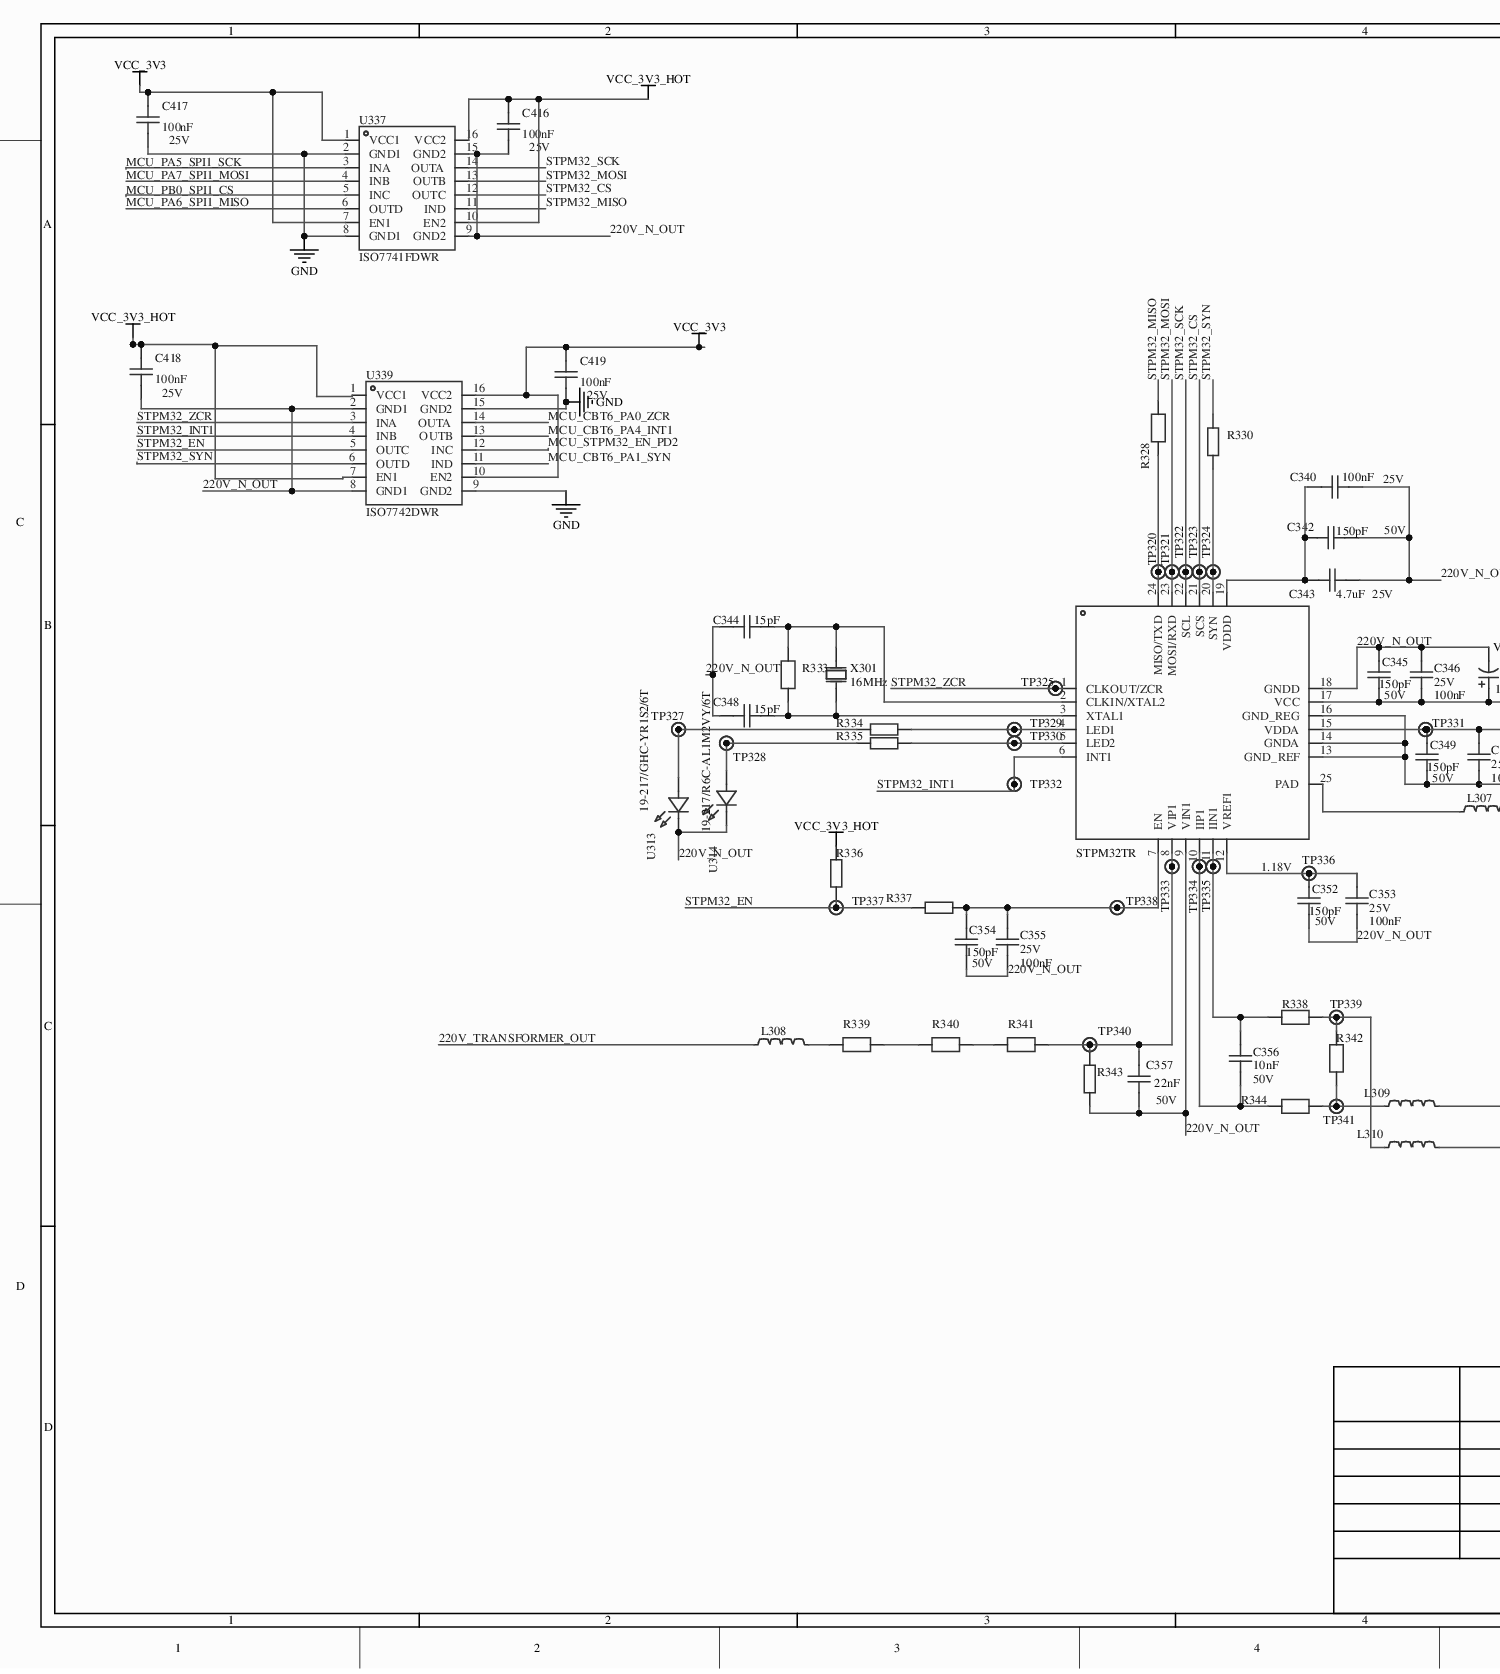
[diagram p0: MISC84429-5.SchDoc, left]
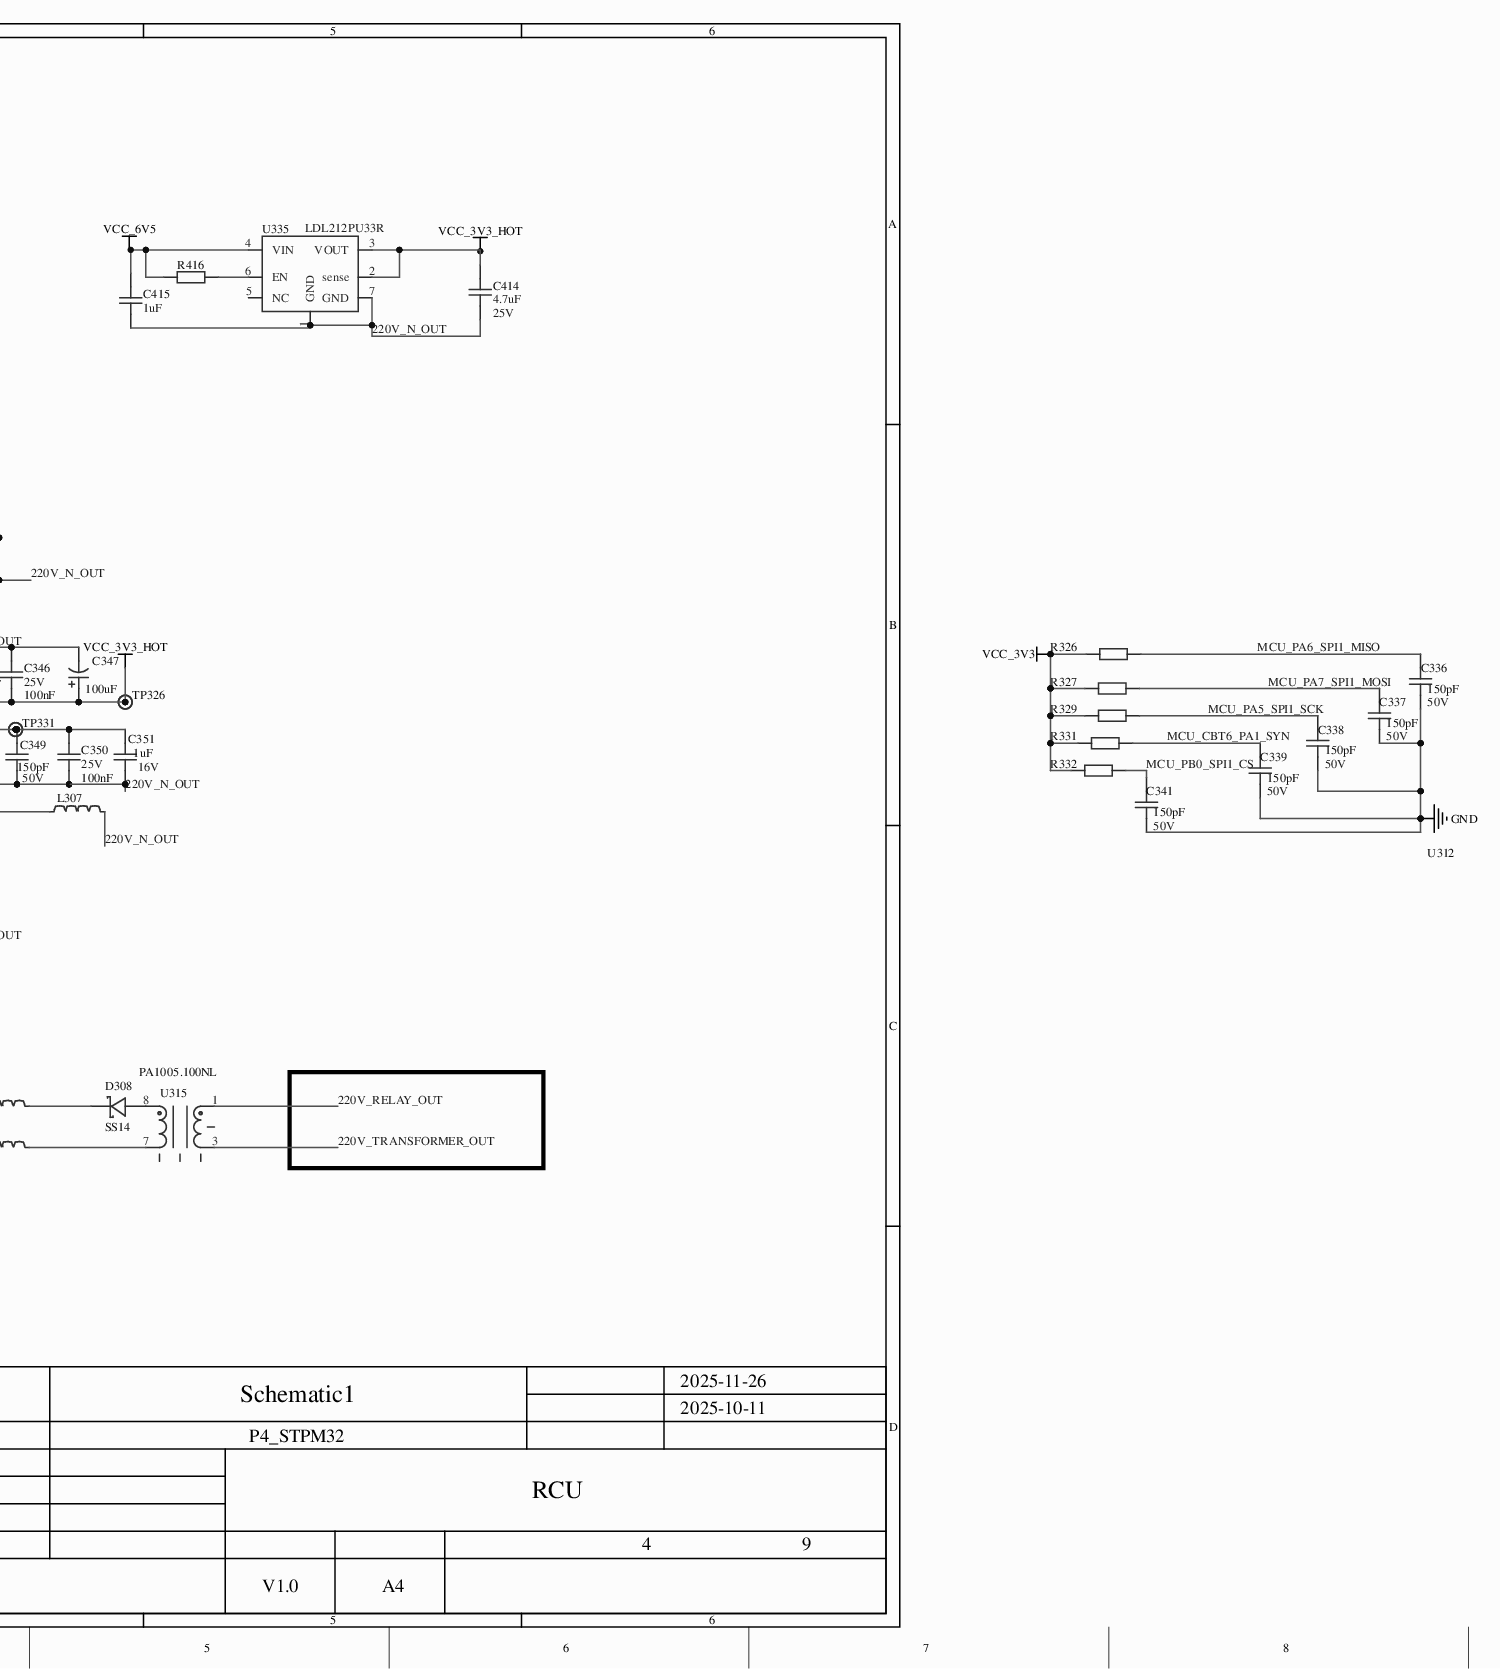
[diagram p1: MISC84429-5.SchDoc, right]
# Altium project MISC84429-12.PrjPcb (part 3 of 5)

## Sheet MISC84429-5.SchDoc
size A1; Name: Sheet-Symbol; Symbol: Sheet-Symbol; Device: Sheet-Symbol; @Page No: 4; @Page Count: 9; @Schematic Name: 1_P1; @Project Name: Altium_Altium_RCU_2025-11-28_2026-01-14; @Board Name: 1_P1; @Update Date: 2026-01-15; @Create Time: 06:40:55; @Update Time: 14:40:57; @Page Name: 4_P4_STPM32; @Create Date: 2026-01-15

### Parts
C336  150pF  Voltage Rating: 50V  [C0603]
C337  150pF  Voltage Rating: 50V  [C0603]
C338  150pF  Voltage Rating: 50V  [C0603]
C339  150pF  Voltage Rating: 50V  [C0603]
C340  100nF  Voltage Rated: 25V  [C0603]
C341  150pF  Voltage Rating: 50V  [C0603]
C342  150pF  Voltage Rating: 50V  [C0603]
C343  4.7uF  Voltage Rating: 25V  [C0603]
C344  15pF  [C0603]
C345  150pF  Voltage Rating: 50V  [C0603]
C346  100nF  Voltage Rated: 25V  [C0603]
C347  100uF  [CAP-SMD_BD6.3-L6.6-W6.6-LS7.3-FD-H7.7]
C348  15pF  [C0603]
C349  150pF  Voltage Rating: 50V  [C0603]
C350  100nF  Voltage Rated: 25V  [C0603]
C351  1uF  Voltage Rated: 16V  [C0603]
C352  150pF  Voltage Rating: 50V  [C0603]
C353  100nF  Voltage Rated: 25V  [C0603]
C354  150pF  Voltage Rating: 50V  [C0603]
C355  100nF  Voltage Rated: 25V  [C0603]
C356  10nF  Voltage Rating: 50V  [C0603]
C357  22nF  Voltage Rating: 50V  [C0805]
C414  4.7uF  Voltage Rating: 25V  [C0603]
C415  1uF  [C0603]
C416  100nF  Voltage Rated: 25V  [C0603]
C417  100nF  Voltage Rated: 25V  [C0603]
C418  100nF  Voltage Rated: 25V  [C0603]
C419  100nF  Voltage Rated: 25V  [C0603]
D308  SS14  [SMA_L4.3-W2.6-LS5.2-RD]
L307  (no value)  [L0805]
L308  (no value)  [L0805]
L309  (no value)  [L0805]
L310  (no value)  [L0805]
R326  (no value)  [R0603]
R327  (no value)  [R0603]
R328  (no value)  [R0603]
R329  (no value)  [R0603]
R330  (no value)  [R0603]
R331  (no value)  [R0603]
R332  (no value)  [R0603]
R333  (no value)  [R0603]
R334  (no value)  [R0603]
R335  (no value)  [R0603]
R336  (no value)  [R0603]
R337  (no value)  [R0603]
R338  (no value)  [R1206]
R339  (no value)  [R1206]
R340  (no value)  [R1206]
R341  (no value)  [R1206]
R342  (no value)  [R1206]
R343  (no value)  [R1206]
R344  (no value)  [R1206]
R416  (no value)  [R0603]
TP320  (no value)  [Test-Point-0.5mm]
TP321  (no value)  [Test-Point-0.5mm]
TP322  (no value)  [Test-Point-0.5mm]
TP323  (no value)  [Test-Point-0.5mm]
TP324  (no value)  [Test-Point-0.5mm]
TP325  (no value)  [Test-Point-0.5mm]
TP326  (no value)  [Test-Point-0.5mm]
TP327  (no value)  [Test-Point-0.5mm]
TP328  (no value)  [Test-Point-0.5mm]
TP329  (no value)  [Test-Point-0.5mm]
TP330  (no value)  [Test-Point-0.5mm]
TP331  (no value)  [Test-Point-0.5mm]
TP332  (no value)  [Test-Point-0.5mm]
TP333  (no value)  [Test-Point-0.5mm]
TP334  (no value)  [Test-Point-0.5mm]
TP335  (no value)  [Test-Point-0.5mm]
TP336  (no value)  [Test-Point-0.5mm]
TP337  (no value)  [Test-Point-0.5mm]
TP338  (no value)  [Test-Point-0.5mm]
TP339  (no value)  [Test-Point-0.5mm]
TP340  (no value)  [Test-Point-0.5mm]
TP341  (no value)  [Test-Point-0.5mm]
U312  STPM32TR  [VQFN-24_L4.0-W4.0-P0.50-BL-EP2.3]
U313  19-217/GHC-YR1S2/6T  [LED0603-RD_GREEN]
U314  19-217/R6C-AL1M2VY/6T  [LED0603-R-FD]
U315  PA1005.100NL  [SENSOR-TH_PA1005.100NL]
U335  LDL212PU33R  [VSON-6_L3.0-W3.0-P0.95-TL-EP_TI_DRP]
U337  ISO7741FDWR  [SOIC-16_L10.3-W7.5-P1.27-LS10.3-BL]
U339  ISO7742DWR  [SOIC-16_L10.3-W7.5-P1.27-LS10.3-BL]
X301  16MHz  [CRYSTAL-SMD_2P-L5.0-W3.2]

### Nets
GND: C336.2 C337.2 C338.2 C339.2 C341.2 C417.2 C419.2 U337.2(GND1) U337.8(GND1) U339.9(GND2) U339.15(GND2)
VCC_3V3: C417.1 C419.1 R326.1 R327.1 R329.1 R331.1 R332.1 U337.1(VCC1) U337.7(EN1) U339.10(EN2) U339.16(VCC2)
VCC_3V3_HOT: C345.1 C346.1 C347.1 C414.2 C416.1 C418.1 R336.2 TP326.1 U312.17(VCC) U335.2(sense) U335.3(VOUT) U337.10(EN2) U337.16(VCC2) U339.1(VCC1) U339.7(EN1)
VCC_6V5: C415.2 R416.1 U335.4(VIN)
220V_N_OUT: C340.2 C342.2 C343.1 C344.1 C345.2 C346.2 C347.2 C348.1 C349.1 C350.1 C351.1 C352.1 C353.1 C354.1 C355.1 C357.1 C414.1 C415.1 C416.2 C418.2 L307.2 R343.1 U312.9(VIN1) U312.13(GND_REF) U312.14(GNDA) U312.16(GND_REG) U312.18(GNDD) U313.1(K) U314.2(K) U335.1(GND) U335.7(GND) U337.9(GND2) U337.15(GND2) U339.2(GND1) U339.8(GND1)
220V_RELAY_OUT: U315.1
220V_TRANSFORMER_OUT: L308.1 U315.3
MCU_CBT6_PA0_ZCR: U339.14(OUTA)
MCU_CBT6_PA1_SYN: C339.1 R331.2 U339.11(IND)
MCU_CBT6_PA4_INT1: U339.13(OUTB)
MCU_PA5_SPI1_SCK: C338.1 R329.2 U337.3(INA)
MCU_PA6_SPI1_MISO: C336.1 R326.2 U337.6(OUTD)
MCU_PA7_SPI1_MOSI: C337.1 R327.2 U337.4(INB)
MCU_PB0_SPI1_CS: C341.1 R332.2 U337.5(INC)
MCU_STPM32_EN_PD2: U339.12(INC)
STPM32_CS: TP323.1 U312.21(SCS) U337.12(OUTC)
STPM32_EN: R336.1 R337.2 TP337.1 U339.5(OUTC)
STPM32_INT1: TP332.1 U312.6(INT1) U339.4(INB)
STPM32_MISO: R328.2 U337.11(IND)
STPM32_MOSI: TP321.1 U312.23(MOSI/RXD) U337.13(OUTB)
STPM32_SCK: TP322.1 U312.22(SCL) U337.14(OUTA)
STPM32_SYN: R330.2 U339.6(OUTD)
STPM32_ZCR: TP325.1 U312.1(CLKOUT/ZCR) U339.3(INA)
NetC340_1: C340.1 C342.1 C343.2 U312.19(VDDD)
NetC344_2: C344.2 R333.2 U312.2(CLKIN/XTAL2) X301.2(OSC2)
NetC348_2: C348.2 R333.1 U312.3(XTAL1) X301.1(OSC1)
NetC349_2: C349.2 C350.2 C351.2 TP331.1 U312.15(VDDA)
NetC352_2: C352.2 C353.2 TP336.1 U312.12(VREF1)
NetC354_2: C354.2 C355.2 R337.1 TP338.1 U312.7(EN)
NetC356_1: C356.1 R344.1 TP334.1 U312.10(IIP1)
NetC356_2: C356.2 R338.1 TP335.1 U312.11(IIN1)
NetC357_2: C357.2 R341.1 R343.2 TP333.1 TP340.1 U312.8(VIP1)
NetD308_1: D308.1(K) L309.2
NetD308_2: D308.2(A) U315.8
NetL307_1: L307.1 U312.25(PAD)
NetL308_2: L308.2 R339.2
NetL309_1: L309.1 R342.1 R344.2 TP341.1
NetL310_1: L310.1 R338.2 R342.2 TP339.1
NetL310_2: L310.2 U315.7
NetR328_1: R328.1 TP320.1 U312.24(MISO/TXD)
NetR330_1: R330.1 TP324.1 U312.20(SYN)
NetR334_1: R334.1 TP327.1 U313.2(A)
NetR334_2: R334.2 TP329.1 U312.4(LED1)
NetR335_1: R335.1 TP328.1 U314.1(A)
NetR335_2: R335.2 TP330.1 U312.5(LED2)
NetR339_1: R339.1 R340.1
NetR340_2: R340.2 R341.2
NetR416_2: R416.2 U335.6(EN)

Not connected (* = marked no-connect by the designer): U315 2* 4* 5* 6*; U335 5(NC)*

### Notes on the sheet
- 1.18V
- 1
- 2
- 3
- 4
- 5
- 6
- A
- B
- C
- D
- Schematic1
- 2025-11-26
- 2025-10-11
- P4_STPM32
- RCU
- 9
- V1.0
- A4

### Library data of the parts
C336-C339 C341 C342 C345 C349 C352 C354 = 150pF: Symbol: GRM1885C1H151JA01D; Add into BOM: yes; Temperature Coefficient: C0G; Device: 150pF; Supplier Part: C85975; Manufacturer Part: GRM1885C1H151JA01D; Supplier Footprint: 0603; Datasheet: https://item.szlcsc.com/datasheet/GRM1885C1H151JA01D/87151.html; Supplier: LCSC; Convert to PCB: yes; Value: 150pF; Origin Footprint: C0603; Design Item ID: GRM1885C1H151JA01D
C340 C346 C350 C353 C355 = 100nF: Symbol: GRM188R71E104KA01D; Add into BOM: yes; Temperature Coefficient: X7R; Device: 100nF; Supplier Part: C77050; Manufacturer Part: GRM188R71E104KA01D; Supplier Footprint: 0603; Datasheet: https://atta.szlcsc.com/upload/public/pdf/source/20170622/1498103881034.pdf; Supplier: LCSC; Convert to PCB: yes; Value: 100nF; Origin Footprint: C0603; Design Item ID: GRM188R71E104KA01D
C343 = 4.7uF: Symbol: GRM188R61E475KE11D; Add into BOM: yes; Temperature Coefficient: X5R; Device: 4.7uF; Supplier Part: C90057; Manufacturer Part: GRM188R61E475KE11D; Supplier Footprint: 0603; Datasheet: https://item.szlcsc.com/datasheet/GRM188R61E475KE11D/91242.html; Supplier: LCSC; Convert to PCB: yes; Value: 4.7uF; Origin Footprint: C0603; Design Item ID: GRM188R61E475KE11D
C344 C348 = 15pF: Symbol: GRM1885C1H150JA01D; Add into BOM: yes; Voltage Rated: 50V; Temperature Coefficient: C0G; Device: 15pF; Supplier Part: C71651; Manufacturer Part: GRM1885C1H150JA01D; Supplier Footprint: 0603; Datasheet: https://atta.szlcsc.com/upload/public/pdf/source/20170116/1484561236820.pdf; Supplier: LCSC; Convert to PCB: yes; Value: 15pF; Origin Footprint: C0603; Design Item ID: GRM1885C1H150JA01D
C347 = 100uF: Symbol: JVJ50V100M6x8; Add into BOM: yes; Voltage Rating: 50V; Ripple Current: 140mA@120Hz; Device: 100uF; Supplier Part: C46550415; Manufacturer Part: JVJ50V100M6x8; Supplier Footprint: SMD,D6.3xL7.7mm; Datasheet: https://item.szlcsc.com/datasheet/JVJ50V100M6x8/48680109.html; Supplier: LCSC; Convert to PCB: yes; Value: 100uF; Diameter: 6.3mm; Height - Seated (Max): 7.7mm; Origin Footprint: CAP-SMD_BD6.3-L6.6-W6.6-LS7.3-FD-H7.7; Design Item ID: JVJ50V100M6x8
C351 = 1uF: Symbol: GCM188R71C105KA64D; Add into BOM: yes; Temperature Coefficient: X7R; Device: 1uF; Supplier Part: C161212; Manufacturer Part: GCM188R71C105KA64D; Supplier Footprint: 0603; Datasheet: https://atta.szlcsc.com/upload/public/pdf/source/20181221/C161212_C96DD77354D5551432B3B7779E4D1948.pdf; Supplier: LCSC; Convert to PCB: yes; Value: 1uF; Origin Footprint: C0603; Design Item ID: GCM188R71C105KA64D
C356 = 10nF: Symbol: GCM188R71H103KA37D; Add into BOM: yes; Temperature Coefficient: X7R; Device: 10nF; Supplier Part: C85863; Manufacturer Part: GCM188R71H103KA37D; Supplier Footprint: 0603; Datasheet: https://item.szlcsc.com/datasheet/GCM188R71H103KA37D/87039.html; Supplier: LCSC; Convert to PCB: yes; Value: 10nF; Origin Footprint: C0603; Design Item ID: GCM188R71H103KA37D
C357 = 22nF: Symbol: GRM21B5C1H223JA01L; Add into BOM: yes; Temperature Coefficient: C0G; Device: 22nF; Supplier Part: C77069; Manufacturer Part: GRM21B5C1H223JA01L; Supplier Footprint: 0805; Datasheet: https://item.szlcsc.com/datasheet/GRM21B5C1H223JA01L/78196.html; Supplier: LCSC; Convert to PCB: yes; Value: 22nF; Origin Footprint: C0805; Design Item ID: GRM21B5C1H223JA01L
C414 = GRM188R61E475KE11D: Add into BOM: yes; Temperature Coefficient: X5R; Symbol: GRM188R61E475KE11D; Device: GRM188R61E475KE11D; Supplier Part: C90057; Manufacturer Part: GRM188R61E475KE11D; Supplier Footprint: 0603; Datasheet: https://item.szlcsc.com/datasheet/GRM188R61E475KE11D/91242.html; Supplier: LCSC; Convert to PCB: yes; Value: 4.7uF
C415 = CGA0603X5R105K500JT: Add into BOM: yes; Voltage Rating: 50V; Temperature Coefficient: X5R; Symbol: CGA0603X5R105K500JT; Device: CGA0603X5R105K500JT; Supplier Part: C6119852; Manufacturer Part: CGA0603X5R105K500JT; Supplier Footprint: 0603; Datasheet: https://item.szlcsc.com/datasheet/CGA0603X5R105K500JT/7062558.html; Supplier: LCSC; Convert to PCB: yes; Value: 1uF
C416-C419 = GRM188R71E104KA01D: Add into BOM: yes; Temperature Coefficient: X7R; Symbol: GRM188R71E104KA01D; Device: GRM188R71E104KA01D; Supplier Part: C77050; Manufacturer Part: GRM188R71E104KA01D; Supplier Footprint: 0603; Datasheet: https://atta.szlcsc.com/upload/public/pdf/source/20170622/1498103881034.pdf; Supplier: LCSC; Convert to PCB: yes; Value: 100nF
D308 = SS14: Symbol: SS14_C83852; Add into BOM: yes; Voltage - Forward(Vf@If): 500mV@1A; Voltage - DC Reverse(Vr): 40V; Current - Rectified: 1A; Reverse Leakage Current (Ir): 200uA@40V; Non-Repetitive Peak Forward Surge Current: 40A; Device: SS14; Supplier Part: C83852; Manufacturer Part: SS14; Supplier Footprint: SMA(DO-214AC); Datasheet: https://item.szlcsc.com/datasheet/SS14/85019.html; Supplier: LCSC; Convert to PCB: yes; Origin Footprint: SMA_L4.3-W2.6-LS5.2-RD; Design Item ID: SS14_C83852
L307-L310 = BLM21BD152SN1D: Add into BOM: yes; Current Rating: 250mA; Circuits: 1; Symbol: BLM21BD152SN1D; Device: BLM21BD152SN1D; Supplier Part: C413959; Supplier Footprint: 0805; Datasheet: https://atta.szlcsc.com/upload/public/pdf/source/20191022/C440135_21EA6A128C5B591010E9DC76809289F4.pdf; Supplier: LCSC; Convert to PCB: yes; Origin Footprint: L0805; Design Item ID: BLM21BD152SN1D
R326 R327 R329 R331 R332 = RC0603FR-0710KL: Add into BOM: yes; Power(Watts): 100mW; Overload Voltage (Max): 75V; Symbol: RC0603FR-0710KL; Device: RC0603FR-0710KL; Supplier Part: C98220; Manufacturer Part: RC0603FR-0710KL; Supplier Footprint: 0603; Datasheet: https://atta.szlcsc.com/upload/public/pdf/source/20180927/C295883_E8D83085EA81BD7DE0B2B681138C15EE.pdf; Supplier: LCSC; Convert to PCB: yes; Origin Footprint: R0603; Design Item ID: RC0603FR-0710KL
R328 = FRC0603F33R0TS: Add into BOM: yes; Power(Watts): 100mW; Voltage-Supply(Max): 75V; Symbol: FRC0603F33R0TS; Device: FRC0603F33R0TS; Supplier Part: C2909394; Manufacturer Part: FRC0603F33R0TS; Supplier Footprint: 0603; Supplier: LCSC; Convert to PCB: yes; Origin Footprint: R0603; Design Item ID: FRC0603F33R0TS
R330 R337 = RC0603FR-07100RL: Add into BOM: yes; Power(Watts): 100mW; Overload Voltage (Max): 75V; Symbol: RC0603FR-07100RL; Device: RC0603FR-07100RL; Supplier Part: C105588; Manufacturer Part: RC0603FR-07100RL; Supplier Footprint: 0603; Datasheet: https://atta.szlcsc.com/upload/public/pdf/source/20180316/70C0E2BDAE7FCC62C531A5A58D202EE1.pdf; Supplier: LCSC; Convert to PCB: yes; Origin Footprint: R0603; Design Item ID: RC0603FR-07100RL
R333 = FRC0603F1004TS: Add into BOM: yes; Power(Watts): 100mW; Voltage-Supply(Max): 75V; Symbol: FRC0603F1004TS; Device: FRC0603F1004TS; Supplier Part: C2907003; Manufacturer Part: FRC0603F1004TS; Supplier Footprint: 0603; Datasheet: https://item.szlcsc.com/datasheet/FRC0603F1004TS/3180516.html; Supplier: LCSC; Convert to PCB: yes; Origin Footprint: R0603; Design Item ID: FRC0603F1004TS
R334 R335 = RC0603FR-07160RL: Add into BOM: yes; Power(Watts): 100mW; Overload Voltage (Max): 75V; Symbol: RC0603FR-07160RL; Device: RC0603FR-07160RL; Supplier Part: C185369; Manufacturer Part: RC0603FR-07160RL; Supplier Footprint: 0603; Datasheet: https://atta.szlcsc.com/upload/public/pdf/source/20180904/C276339_014E484F1DBA106FB92D45EABD5A1AC1.pdf; Supplier: LCSC; Convert to PCB: yes; Origin Footprint: R0603; Design Item ID: RC0603FR-07160RL
R336 = RC0603FR-0722KL: Add into BOM: yes; Power(Watts): 100mW; Voltage-Supply(Max): 75V; Symbol: RC0603FR-0722KL; Device: RC0603FR-0722KL; Supplier Part: C114065; Manufacturer Part: RC0603FR-0722KL; Supplier Footprint: 0603; Datasheet: https://item.szlcsc.com/datasheet/RC0603FR-0722KL/115304.html; Supplier: LCSC; Convert to PCB: yes; Origin Footprint: R0603; Design Item ID: RC0603FR-0722KL
R338 R344 = FRC1206F1001TS: Add into BOM: yes; Power(Watts): 250mW; Voltage-Supply(Max): 200V; Symbol: FRC1206F1001TS; Device: FRC1206F1001TS; Supplier Part: C2907372; Manufacturer Part: FRC1206F1001TS; Supplier Footprint: 1206; Supplier: LCSC; Convert to PCB: yes; Origin Footprint: R1206; Design Item ID: FRC1206F1001TS
R339-R341 = FRC1206F2703TS: Add into BOM: yes; Power(Watts): 250mW; Voltage-Supply(Max): 200V; Symbol: FRC1206F2703TS; Device: FRC1206F2703TS; Supplier Part: C2960856; Manufacturer Part: FRC1206F2703TS; Supplier Footprint: 1206; Supplier: LCSC; Convert to PCB: yes; Origin Footprint: R1206; Design Item ID: FRC1206F2703TS
R342 = PA1206FRF470R05L: Add into BOM: yes; Power(Watts): 1W; Symbol: PA1206FRF470R05L; Device: PA1206FRF470R05L; Supplier Part: C728294; Manufacturer Part: PA1206FRF470R05L; Supplier Footprint: 1206; Datasheet: https://atta.szlcsc.com/upload/public/pdf/source/20201130/C728294_18A3BD30D8B965C3DA67B18223572289.pdf; Supplier: LCSC; Convert to PCB: yes; Origin Footprint: R1206; Design Item ID: PA1206FRF470R05L
R343 = RC1206JR-07470RL: Add into BOM: yes; Power(Watts): 250mW; Voltage-Supply(Max): 200V; Symbol: RC1206JR-07470RL; Device: RC1206JR-07470RL; Supplier Part: C114948; Manufacturer Part: RC1206JR-07470RL; Supplier Footprint: 1206; Datasheet: https://item.szlcsc.com/datasheet/RC1206JR-07470RL/116192.html; Supplier: LCSC; Convert to PCB: yes; Origin Footprint: R1206; Design Item ID: RC1206JR-07470RL
R416 = 0603WAF1002T5E: Add into BOM: yes; Power(Watts): 100mW; Voltage-Supply(Max): 75V; Symbol: 0603WAF1002T5E; Device: 0603WAF1002T5E; Supplier Part: C25804; Manufacturer Part: 0603WAF1002T5E; Supplier Footprint: 0603; Datasheet: https://item.szlcsc.com/datasheet/0603WAF1002T5E/26547.html; Supplier: LCSC; Convert to PCB: yes
TP320-TP341 = Test-Point: Add into BOM: yes; Symbol: Test-Point; Device: Test-Point; Convert to PCB: yes; Origin Footprint: Test-Point-0.5mm; Design Item ID: Test-Point
U312 = STPM32TR: Add into BOM: yes; Number of Channels: 4; Voltage - Supply: 2.95V~3.65V; Dynamic Range: 5000:1; Current - Supply: 4.3mA; Symbol: STPM32TR; Device: STPM32TR; LCSC Part Name: STPM32TR; Supplier Part: C128380; Manufacturer Part: STPM32TR; Supplier Footprint: QFN-24-EP(4x4); Datasheet: https://item.szlcsc.com/datasheet/STPM32TR/139665.html; Supplier: LCSC; Convert to PCB: yes; Origin Footprint: VQFN-24_L4.0-W4.0-P0.50-BL-EP2.3; Design Item ID: STPM32TR
U313 = 19-217/GHC-YR1S2/6T: Add into BOM: yes; Symbol: 19-217/GHC-YR1S2/6T; Device: 19-217/GHC-YR1S2/6T; Supplier Part: C2986059; Manufacturer Part: 19-217/GHC-YR1S2/6T; Supplier Footprint: 0603; Datasheet: https://atta.szlcsc.com/upload/public/pdf/source/20220705/5270194960AA522E2931401D212035CB.pdf; Supplier: LCSC; Convert to PCB: yes; Origin Footprint: LED0603-RD_GREEN; Design Item ID: 19-217/GHC-YR1S2/6T
U314 = 19-217/R6C-AL1M2VY/6T: Add into BOM: yes; Symbol: 19-217/R6C-AL1M2VY/6T; Device: 19-217/R6C-AL1M2VY/6T; LCSC Part Name: 19-217/R6C-AL1M2VY/6T; Supplier Part: C2986060; Manufacturer Part: 19-217/R6C-AL1M2VY/6T; Supplier Footprint: 0603; Datasheet: https://www.everlighteurope.com/custom/files/datasheets/DSE-0014128.pdf; Supplier: LCSC; Convert to PCB: yes; Lamp Holder Type: -; Voltage - Forward(Vf): -; Power(Watts): -; Forward Current: -; Wavelength - Dominant: -; Peak Wavelength: -; Diode Configuration: -; Lens Color: -; Color Temperature: -; Luminous Intensity: -; Viewing Angle: -; Mounting Style: -; Operating Temperature: -; Origin Footprint: LED0603-R-FD; Design Item ID: 19-217/R6C-AL1M2VY/6T
U315 = PA1005.100NL: Add into BOM: yes; Isolation Voltage(Vrms): 1000Vrms; Symbol: PA1005.100NL; Device: PA1005.100NL; LCSC Part Name: PA1005.100NL; Supplier Part: C428625; Manufacturer Part: PA1005.100NL; Supplier Footprint: SMD-8P,8.4x7.2mm; Datasheet: https://item.szlcsc.com/datasheet/PA1005.100NL/423576.html; Supplier: LCSC; Convert to PCB: yes; Origin Footprint: SENSOR-TH_PA1005.100NL; Design Item ID: PA1005.100NL
U335 = LDL212PU50R: Add into BOM: yes; Maximum Input Voltage: 18V; Output Voltage: 5V; Output Current: 1.2A; Power Supply Rejection Ratio (PSRR): 87dB@(120Hz); Symbol: LDL212PU50R; Device: LDL212PU50R; Supplier Part: C2761339; Manufacturer Part: LDL212PU33R; Supplier Footprint: DFN-6-EP(3x3); Datasheet: https://atta.szlcsc.com/upload/public/pdf/source/20240527/4417E89F3C8FA1CE0333A3FDFF72E004.pdf; Supplier: LCSC; Convert to PCB: yes
U337 = ISO7741FDWR: Add into BOM: yes; Number of Forward Channels: 3; Number of Reverse Channels: 1; Data Rate(Max): 100Mbps; Isolation Voltage(Vrms): 5000; CMTI(kV/us): 100kV/us; Symbol: ISO7741FDWR; Device: ISO7741FDWR; LCSC Part Name: ISO7741FDWR; Supplier Part: C485810; Manufacturer Part: ISO7741FDWR; Supplier Footprint: SOIC-16-300mil; Datasheet: https://www.ti.com/cn/lit/gpn/iso7741; Supplier: LCSC; Convert to PCB: yes
U339 = ISO7742DWR: Add into BOM: yes; Number of Forward Channels: 2; Data Rate(Max): 100Mbps; Isolation Voltage(Vrms): 5000; CMTI(kV/us): 100kV/us; Voltage - Supply(VCCA): 2.25V~5.5V; Propagation Delay(tpd): 10.7ns; Symbol: ISO7742DWR; Device: ISO7742DWR; Supplier Part: C529288; Manufacturer Part: ISO7742DWR; Supplier Footprint: SOIC-16-300mil; Datasheet: https://www.ti.com/cn/lit/gpn/iso7740; Supplier: LCSC; Convert to PCB: yes; Number of Reverse Channels: 2; Voltage - Supply(VCCB): 2.25V~5.5V
X301 = 16MHz: Symbol: XG1EL89CSI-111YLC-16M; Add into BOM: yes; Load Capacitance: 20pF; Device: 16MHz; Supplier Part: C7528816; Manufacturer Part: XG1EL89CSI-111YLC-16M; Supplier Footprint: SMD5032-2P; Datasheet: https://item.szlcsc.com/datasheet/XG1EL89CSI-111YLC-16M/8628156.html; Supplier: LCSC; Convert to PCB: yes; Value: 16MHz; Origin Footprint: CRYSTAL-SMD_2P-L5.0-W3.2; Design Item ID: XG1EL89CSI-111YLC-16M

## Sheet MISC84429-6.SchDoc
size 431 x 309 mm; Name: Sheet-Symbol; Symbol: Sheet-Symbol; Device: Sheet-Symbol
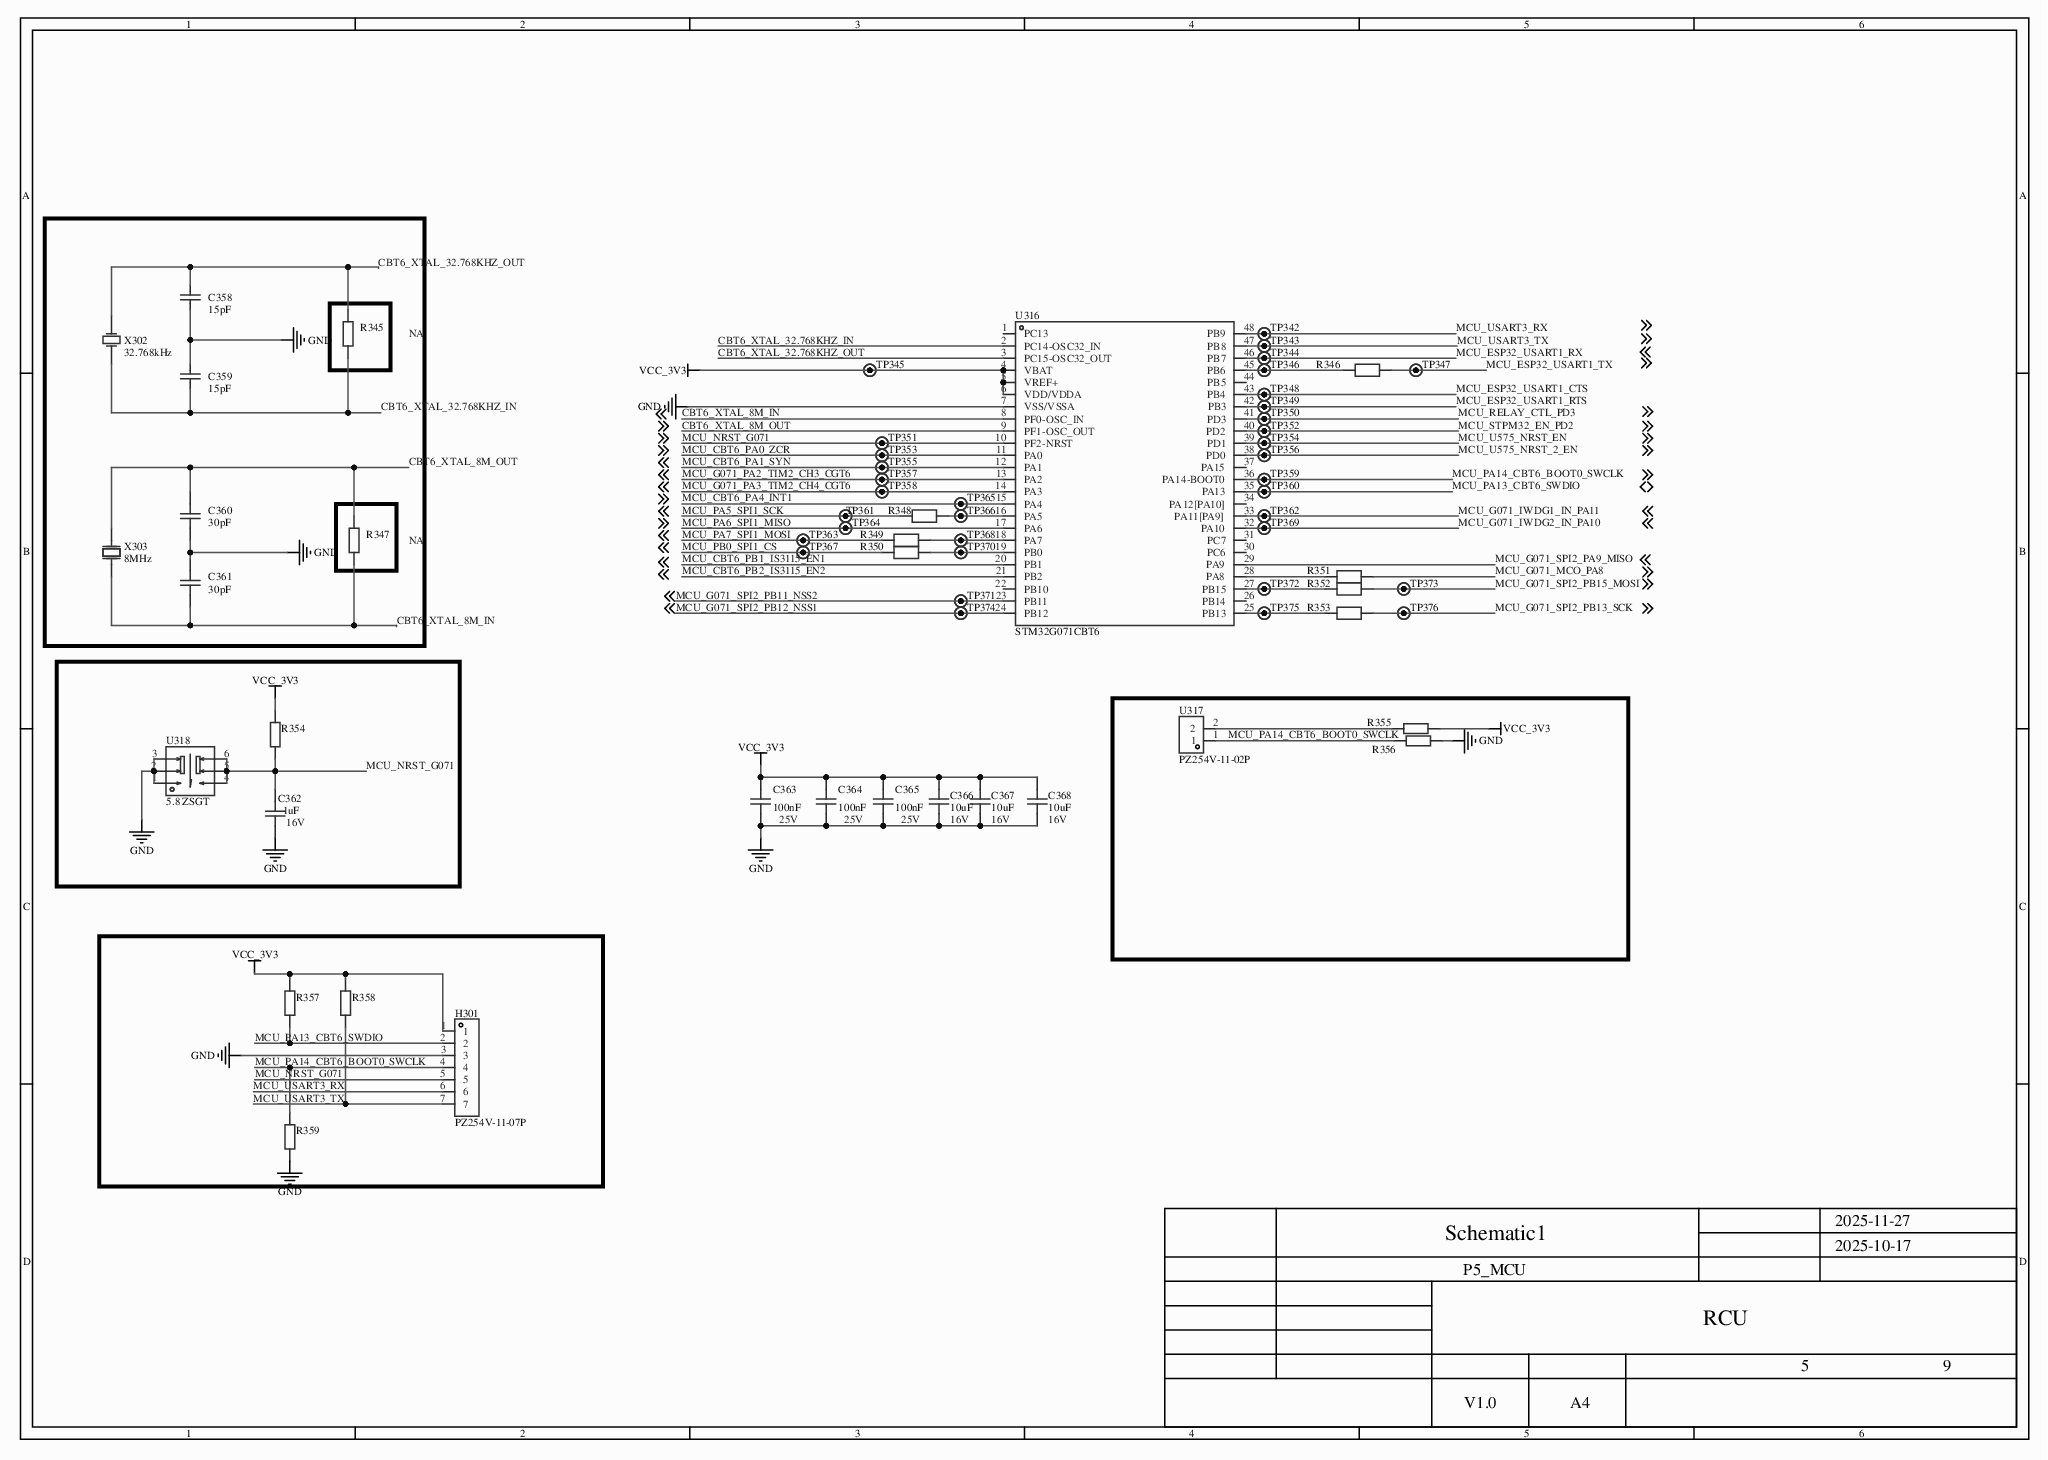
[diagram p2: MISC84429-6.SchDoc]

### Parts
C358  15pF  [C0402]
C359  15pF  [C0402]
C360  30pF  [C0402]
C361  30pF  [C0402]
C362  1uF  Voltage Rated: 16V  [C0603]
C363  100nF  Voltage Rated: 25V  [C0603]
C364  100nF  Voltage Rated: 25V  [C0603]
C365  100nF  Voltage Rated: 25V  [C0603]
C366  10uF  Voltage Rated: 16V  [C0805]
C367  10uF  Voltage Rated: 16V  [C0805]
C368  10uF  Voltage Rated: 16V  [C0805]
H301  PZ254V-11-07P  [HDR-TH_7P-P2.54-V-M]
R345  (no value)  [R0402]
R346  (no value)  [R0603]
R347  (no value)  [R0402]
R348  (no value)  [R0603]
R349  (no value)  [R0603]
R350  (no value)  [R0603]
R351  (no value)  [R0603]
R352  (no value)  [R0603]
R353  (no value)  [R0603]
R354  (no value)  [R0603]
R355  (no value)  [R0603]
R356  (no value)  [R0603]
R357  (no value)  [R0603]
R358  (no value)  [R0603]
R359  (no value)  [R0603]
TP342  (no value)  [Test-Point-0.5mm]
TP343  (no value)  [Test-Point-0.5mm]
TP344  (no value)  [Test-Point-0.5mm]
TP345  (no value)  [Test-Point-0.5mm]
TP346  (no value)  [Test-Point-0.5mm]
TP347  (no value)  [Test-Point-0.5mm]
TP348  (no value)  [Test-Point-0.5mm]
TP349  (no value)  [Test-Point-0.5mm]
TP350  (no value)  [Test-Point-0.5mm]
TP351  (no value)  [Test-Point-0.5mm]
TP352  (no value)  [Test-Point-0.5mm]
TP353  (no value)  [Test-Point-0.5mm]
TP354  (no value)  [Test-Point-0.5mm]
TP355  (no value)  [Test-Point-0.5mm]
TP356  (no value)  [Test-Point-0.5mm]
TP357  (no value)  [Test-Point-0.5mm]
TP358  (no value)  [Test-Point-0.5mm]
TP359  (no value)  [Test-Point-0.5mm]
TP360  (no value)  [Test-Point-0.5mm]
TP361  (no value)  [Test-Point-0.5mm]
TP362  (no value)  [Test-Point-0.5mm]
TP363  (no value)  [Test-Point-0.5mm]
TP364  (no value)  [Test-Point-0.5mm]
TP365  (no value)  [Test-Point-0.5mm]
TP366  (no value)  [Test-Point-0.5mm]
TP367  (no value)  [Test-Point-0.5mm]
TP368  (no value)  [Test-Point-0.5mm]
TP369  (no value)  [Test-Point-0.5mm]
TP370  (no value)  [Test-Point-0.5mm]
TP371  (no value)  [Test-Point-0.5mm]
TP372  (no value)  [Test-Point-0.5mm]
TP373  (no value)  [Test-Point-0.5mm]
TP374  (no value)  [Test-Point-0.5mm]
TP375  (no value)  [Test-Point-0.5mm]
TP376  (no value)  [Test-Point-0.5mm]
U316  STM32G071CBT6  [LQFP-48_L7.0-W7.0-P0.50-LS9.0-BL]
U317  PZ254V-11-02P  [HDR-TH_2P-P2.54-V-M]
U318  5.8 ZSGT  [SW-TH_5.8ZSGT]
X302  32.768kHz  [OSC-TH_BD3.1-P0.8-D0.3]
X303  8MHz  [CRYSTAL-SMD_L5.0-W3.2]

### Nets
GND: C358.1 C359.2 C360.2 C361.1 C362.1 C363.2 C364.2 C365.2 C366.1 C367.1 C368.1 H301.3 R356.2 R359.2 U316.7(VSS/VSSA) U318.1 U318.2 U318.3
VCC_3V3: C363.1 C364.1 C365.1 C366.2 C367.2 C368.2 H301.1 R354.2 R355.2 R357.2 R358.2 TP345.1 U316.4(VBAT) U316.5(VREF+) U316.6(VDD/VDDA)
CBT6_XTAL_8M_IN: C361.2 R347.1 U316.8(PF0-OSC_IN) X303.1(OSC1)
CBT6_XTAL_8M_OUT: C360.1 R347.2 U316.9(PF1-OSC_OUT) X303.2(OSC2)
CBT6_XTAL_32.768KHZ_IN: C359.1 R345.1 U316.2(PC14-OSC32_IN) X302.1(OSC1)
CBT6_XTAL_32.768KHZ_OUT: C358.2 R345.2 U316.3(PC15-OSC32_OUT) X302.2(OSC2)
MCU_CBT6_PA0_ZCR: TP353.1 U316.11(PA0)
MCU_CBT6_PA1_SYN: TP355.1 U316.12(PA1)
MCU_CBT6_PA4_INT1: TP365.1 U316.15(PA4)
MCU_CBT6_PB1_IS3115_EN1: U316.20(PB1)
MCU_CBT6_PB2_IS3115_EN2: U316.21(PB2)
MCU_ESP32_USART1_CTS: TP348.1 U316.43(PB4)
MCU_ESP32_USART1_RTS: TP349.1 U316.42(PB3)
MCU_ESP32_USART1_RX: TP344.1 U316.46(PB7)
MCU_ESP32_USART1_TX: R346.1 TP347.1
MCU_G071_IWDG1_IN_PA11: TP362.1 U316.33(PA11[PA9])
MCU_G071_IWDG2_IN_PA10: TP369.1 U316.32(PA10)
MCU_G071_MCO_PA8: R351.1
MCU_G071_PA2_TIM2_CH3_CGT6: TP357.1 U316.13(PA2)
MCU_G071_PA3_TIM2_CH4_CGT6: TP358.1 U316.14(PA3)
MCU_G071_SPI2_PA9_MISO: U316.29(PA9)
MCU_G071_SPI2_PB11_NSS2: TP371.1 U316.23(PB11)
MCU_G071_SPI2_PB12_NSS1: TP374.1 U316.24(PB12)
MCU_G071_SPI2_PB13_SCK: R353.1 TP376.1
MCU_G071_SPI2_PB15_MOSI: R352.1 TP373.1
MCU_NRST_G071: C362.2 H301.5 R354.1 TP351.1 U316.10(PF2-NRST) U318.4 U318.5 U318.6
MCU_PA5_SPI1_SCK: R348.2 TP361.1
MCU_PA6_SPI1_MISO: TP364.1 U316.17(PA6)
MCU_PA7_SPI1_MOSI: R349.2 TP363.1
MCU_PA13_CBT6_SWDIO: H301.2 R357.1 TP360.1 U316.35(PA13)
MCU_PA14_CBT6_BOOT0_SWCLK: H301.4 R356.1 R359.1 TP359.1 U316.36(PA14-BOOT0) U317.1
MCU_PB0_SPI1_CS: R350.2 TP367.1
MCU_RELAY_CTL_PD3: TP350.1 U316.41(PD3)
MCU_STPM32_EN_PD2: TP352.1 U316.40(PD2)
MCU_U575_NRST_2_EN: TP356.1 U316.38(PD0)
MCU_U575_NRST_EN: TP354.1 U316.39(PD1)
MCU_USART3_RX: H301.6 TP342.1 U316.48(PB9)
MCU_USART3_TX: H301.7 R358.1 TP343.1 U316.47(PB8)
NetR346_2: R346.2 TP346.1 U316.45(PB6)
NetR348_1: R348.1 TP366.1 U316.16(PA5)
NetR349_1: R349.1 TP368.1 U316.18(PA7)
NetR350_1: R350.1 TP370.1 U316.19(PB0)
NetR351_2: R351.2 U316.28(PA8)
NetR352_2: R352.2 TP372.1 U316.27(PB15)
NetR353_2: R353.2 TP375.1 U316.25(PB13)
NetR355_1: R355.1 U317.2

Not connected (* = marked no-connect by the designer): U316 1(PC13)* 22(PB10)* 26(PB14)* 30(PC6)* 31(PC7)* 34(PA12[PA10])* 37(PA15)* 44(PB5)*

### Notes on the sheet
- NA
- 1
- 2
- 3
- 4
- 5
- 6
- A
- B
- C
- D
- Schematic1
- 2025-11-27
- 2025-10-17
- P5_MCU
- RCU
- 9
- V1.0
- A4

### Library data of the parts
C358 C359 = GJM1555C1H150FB01D: Add into BOM: yes; Voltage Rated: 50V; Temperature Coefficient: C0G; Symbol: GJM1555C1H150FB01D; Device: GJM1555C1H150FB01D; Supplier Part: C441742; Manufacturer Part: GJM1555C1H150FB01D; Supplier Footprint: 0402; Datasheet: https://atta.szlcsc.com/upload/public/pdf/source/20200305/C490387_23319AE8C154DEB24C505E6C82A8106A.pdf; Supplier: LCSC; Convert to PCB: yes; Value: 15pF; Origin Footprint: C0402
C360 C361 = GJM1555C1H300FB01D: Add into BOM: yes; Voltage Rated: 50V; Temperature Coefficient: C0G; Symbol: GJM1555C1H300FB01D; Device: GJM1555C1H300FB01D; Supplier Part: C882565; Manufacturer Part: GJM1555C1H300FB01D; Supplier Footprint: 0402; Datasheet: https://atta.szlcsc.com/upload/public/pdf/source/20201204/C882565_9B5FF39E942C7DB129C3C8F94C41DD81.pdf; Supplier: LCSC; Convert to PCB: yes; Value: 30pF; Origin Footprint: C0402
C362 = GCM188R71C105KA64D: Add into BOM: yes; Temperature Coefficient: X7R; Symbol: GCM188R71C105KA64D; Device: GCM188R71C105KA64D; Supplier Part: C161212; Manufacturer Part: GCM188R71C105KA64D; Supplier Footprint: 0603; Datasheet: https://atta.szlcsc.com/upload/public/pdf/source/20181221/C161212_C96DD77354D5551432B3B7779E4D1948.pdf; Supplier: LCSC; Convert to PCB: yes; Value: 1uF; Origin Footprint: C0603
C363-C365 = GRM188R71E104KA01D: as C416-C419 on sheet MISC84429-5; Symbol: GRM188R71E104KA01D; Device: GRM188R71E104KA01D; Supplier Part: C77050; Manufacturer Part: GRM188R71E104KA01D; Supplier Footprint: 0603; Datasheet: https://atta.szlcsc.com/upload/public/pdf/source/20170622/1498103881034.pdf; Supplier: LCSC; Convert to PCB: yes; Value: 100nF; Origin Footprint: C0603
C366-C368 = GRM21BR61C106KE15L: Add into BOM: yes; Temperature Coefficient: X5R; Symbol: GRM21BR61C106KE15L; Device: GRM21BR61C106KE15L; Supplier Part: C77075; Manufacturer Part: GRM21BR61C106KE15L; Supplier Footprint: 0805; Datasheet: https://atta.szlcsc.com/upload/public/pdf/source/20200305/C490387_23319AE8C154DEB24C505E6C82A8106A.pdf; Supplier: LCSC; Convert to PCB: yes; Value: 10uF; Origin Footprint: C0805
H301 = PZ254V-11-07P: Add into BOM: yes; Pin Structure: 1x7P; Pitch: 2.54mm; Symbol: PZ254V-11-07P; Device: PZ254V-11-07P; Supplier Part: C492406; Manufacturer Part: PZ254V-11-07P; Datasheet: https://atta.szlcsc.com/upload/public/pdf/source/20200309/C492406_654C533EE691117E22DD9F76C114C2D9.pdf; Supplier: LCSC; Convert to PCB: yes; Row Spacing: -; Number of Pins: 7P; Current Rating: -; Voltage Rating (Max): -; Length of Mating Pin: 6mm; Insulation Height: 2.5mm; Length of End Connection Pin: 3mm; Contact Plating: -; Origin Footprint: HDR-TH_7P-P2.54-V-M
R345 = 0402WGF1002TCE: Add into BOM: yes; Power(Watts): 62.5mW; Overload Voltage (Max): 50V; Symbol: 0402WGF1002TCE; Device: 0402WGF1002TCE; Supplier Part: C25744; Manufacturer Part: 0402WGF1002TCE; Supplier Footprint: 0402; Datasheet: https://atta.szlcsc.com/upload/public/pdf/source/20200306/C422600_1E6D84923E4A46A82E41ADD87F860B5C.pdf; Supplier: LCSC; Convert to PCB: yes; Origin Footprint: R0402
R346 R348-R353 = FRC0603F33R0TS: as R328 on sheet MISC84429-5; Symbol: FRC0603F33R0TS; Device: FRC0603F33R0TS; Supplier Part: C2909394; Manufacturer Part: FRC0603F33R0TS; Supplier Footprint: 0603; Supplier: LCSC; Convert to PCB: yes; Origin Footprint: R0603
R347 = 0402WGF1004TCE: Add into BOM: yes; Power(Watts): 62.5mW; Overload Voltage (Max): 50V; Symbol: 0402WGF1004TCE; Device: 0402WGF1004TCE; Supplier Part: C26083; Manufacturer Part: 0402WGF1004TCE; Supplier Footprint: 0402; Datasheet: https://atta.szlcsc.com/upload/public/pdf/source/20200306/C422600_1E6D84923E4A46A82E41ADD87F860B5C.pdf; Supplier: LCSC; Convert to PCB: yes; Origin Footprint: R0402
R354 R356-R359 = RC0603FR-0710KL: as R326 on sheet MISC84429-5; Symbol: RC0603FR-0710KL; Device: RC0603FR-0710KL; Supplier Part: C98220; Manufacturer Part: RC0603FR-0710KL; Supplier Footprint: 0603; Datasheet: https://atta.szlcsc.com/upload/public/pdf/source/20180927/C295883_E8D83085EA81BD7DE0B2B681138C15EE.pdf; Supplier: LCSC; Convert to PCB: yes; Origin Footprint: R0603
R355 = RC0603FR-07100KL: Add into BOM: yes; Power(Watts): 100mW; Overload Voltage (Max): 75V; Symbol: RC0603FR-07100KL; Device: RC0603FR-07100KL; Supplier Part: C14675; Manufacturer Part: RC0603FR-07100KL; Supplier Footprint: 0603; Datasheet: https://atta.szlcsc.com/upload/public/pdf/source/20140324/1457707028752.pdf; Supplier: LCSC; Convert to PCB: yes; Origin Footprint: R0603
TP342-TP376 = Test-Point: Add into BOM: yes; Symbol: Test-Point; Device: Test-Point; Convert to PCB: yes; Origin Footprint: Test-Point-0.5mm
U316 = STM32G071CBT6: Add into BOM: yes; CPU Core: ARM-M0+; CPU Maximum Speed: 64MHz; Program Storage Size: 128KB; Program Memory Type: FLASH; Number of I/O: 44; ADC (Bit): 12bit; Voltage - Supply: 1.71V~3.6V; Symbol: STM32G071CBT6; Device: STM32G071CBT6; Supplier Part: C432212; Manufacturer Part: STM32G071CBT6; Supplier Footprint: LQFP-48(7x7); Datasheet: https://item.szlcsc.com/datasheet/STM32G071CBT6/429000.html; Supplier: LCSC; Convert to PCB: yes; DAC (Bit): 12bit; Applications: -; Origin Footprint: LQFP-48_L7.0-W7.0-P0.50-LS9.0-BL
U317 = PZ254V-11-02P: Add into BOM: yes; Pin Structure: 1x2P; Pitch: 2.54mm; Symbol: PZ254V-11-02P; Device: PZ254V-11-02P; Supplier Part: C492401; Manufacturer Part: PZ254V-11-02P; Datasheet: https://atta.szlcsc.com/upload/public/pdf/source/20200309/C492401_A812433581A9B211A7FFA413ADDFF0E5.pdf; Supplier: LCSC; Convert to PCB: yes; Row Spacing: -; Number of Pins: 2P; Current Rating (Max): -; Voltage Rating (Max): -; Length of Mating Pin: 6mm; Insulation Height: 2.5mm; Length of End Connection Pin: 3mm; Contact Plating: -; Origin Footprint: HDR-TH_2P-P2.54-V-M
U318 = 5.8 ZSGT: Add into BOM: yes; Contact Current: 110mA; Voltage Rating (DC): 30V; Operating Force: 1.5N; Symbol: 5.8 ZSGT; Device: 5.8 ZSGT; Supplier Part: C2681587; Manufacturer Part: 5.8 ZSGT; Datasheet: https://atta.szlcsc.com/upload/public/pdf/source/20210107/C2681587_CDDDDA4A1C7AC9FEB01815B75893A6BA.pdf; Supplier: LCSC; Convert to PCB: yes; Origin Footprint: SW-TH_5.8ZSGT
X302 = X308032768KGB2SC: Add into BOM: yes; Load Capacitance: 12.5pF; Symbol: X308032768KGB2SC; Device: X308032768KGB2SC; Supplier Part: C52082; Manufacturer Part: X308032768KGB2SC; Supplier Footprint: DT-38; Datasheet: https://item.szlcsc.com/datasheet/X308032768KGB2SC/53096.html; Supplier: LCSC; Convert to PCB: yes; Value: 32.768kHz; Origin Footprint: OSC-TH_BD3.1-P0.8-D0.3
X303 = X50328MSB2GI: Add into BOM: yes; Load Capacitor: 20pF; Symbol: X50328MSB2GI; Device: X50328MSB2GI; Supplier Part: C115962; Manufacturer Part: X50328MSB2GI; Supplier Footprint: SMD5032; Datasheet: https://atta.szlcsc.com/upload/public/pdf/source/20240329/44922B0AF7B60E58E9B66993B6077277.pdf; Supplier: LCSC; Convert to PCB: yes; Value: 8MHz; Origin Footprint: CRYSTAL-SMD_L5.0-W3.2